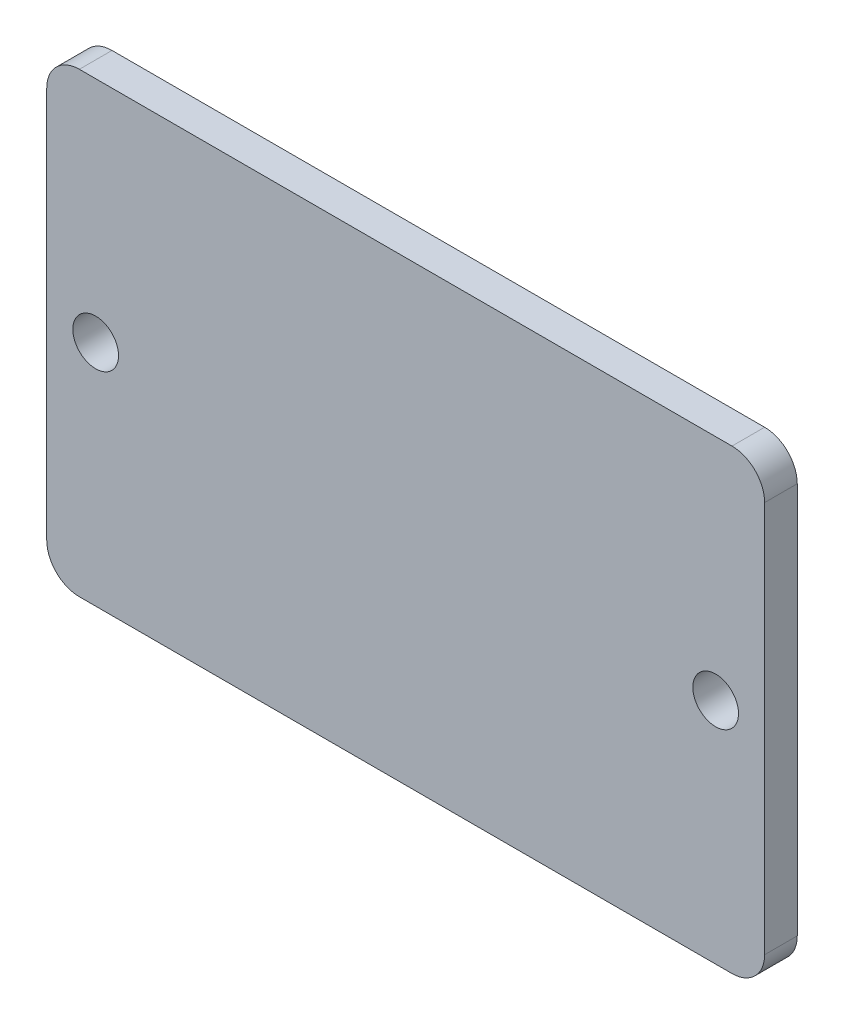
SolidWorks part; units mm, degrees
material "Q235"
ref_plane "Front Plane" through (0, 0, 0) normal (0, 0, 1) x (1, 0, 0)
ref_plane "Top Plane" through (0, 0, 0) normal (0, 1, 0) x (1, 0, 0)
ref_plane "Right Plane" through (0, 0, 0) normal (1, 0, 0) x (0, 0, -1)
sketch "Sketch1" plane through (0, 0, 0) normal (0, 0, 1) x (1, 0, 0)
  line L0 (-95, 0) -> (-110, 0) construction
  line L1 (-110, -70) -> (110, -70)
  line L2 (-110, -70) -> (-110, 70)
  line L3 (-110, 70) -> (110, 70)
  line L4 (110, -70) -> (110, 70)
  line L5 (-95, 0) -> (95, 0) construction
  line L6 (95, 0) -> (110, 0) construction
  line L7 (0, 0) -> (0, 70) construction
  circle A0 centre (-95, 0) radius 7
  circle A1 centre (95, 0) radius 7
  dimension "D3" = 14
  dimension "D4" = 190
  dimension "D1" = 140
  dimension "D2" = 220
extrude "Boss-Extrude1" add sketch "Sketch1" along normal blind 10
fillet "Fillet1" radius 10 4 edges at (110, -70, 5) (-110, -70, 5) (110, 70, 5) (-110, 70, 5)
